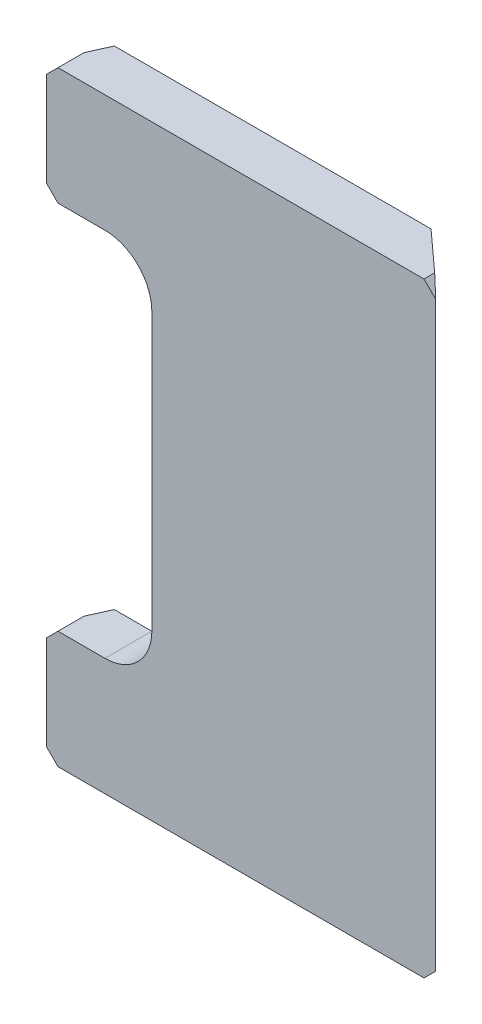
from build123d import *

# Parameters (mm, degrees)
BOSS_EXTRUDE1_DEPTH = 20
CUT_EXTRUDE1_DEPTH  = 308.44105126


with BuildPart() as part:
    # Sketch1 → Boss-Extrude1 (new body)
    with BuildSketch(Plane.XY):
        with BuildLine():
            Line((45, 188), (45, 70))
            ThreePointArc((45, 70), (39.142135624, 55.857864376), (25, 50))
            Line((25, 50), (5, 50))
            Line((5, 50), (0, 45))
            Line((0, 45), (0, 5))
            Line((0, 5), (5, 0))
            Line((5, 0), (161, 0))
            Line((161, 0), (166, 5))
            Line((166, 5), (166, 253))
            Line((166, 253), (161, 258))
            Line((161, 258), (5, 258))
            Line((5, 258), (0, 253))
            Line((0, 253), (0, 213))
            Line((0, 213), (5, 208))
            Line((5, 208), (25, 208))
            ThreePointArc((25, 208), (39.142135624, 202.142135624), (45, 188))
        make_face()
    extrude(amount=BOSS_EXTRUDE1_DEPTH)

    # Sketch2 → Cut-Extrude1 (cut, through all)
    with BuildSketch(Plane.XZ):
        Polygon((0, 20), (0, 0), (9, 0), align=None)
        Polygon((166, 20), (166, 0), (144, 0), align=None)
    extrude(amount=-CUT_EXTRUDE1_DEPTH, mode=Mode.SUBTRACT)


solid = part.part
